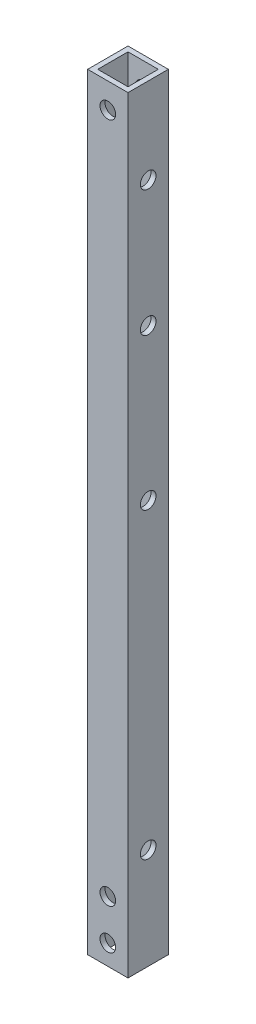
from build123d import *

# Parameters (mm, degrees)
SKETCH_1_W          = 8
SKETCH_1_H          = 8
SKETCH_1_W_2        = 6
SKETCH_1_H_2        = 6
EXTRUDE_1_DEPTH     = 152
SKETCH_2_R          = 1.55
CUT_EXTRUDE_1_DEPTH = 153.262930485
SKETCH_3_R          = 1.55
CUT_EXTRUDE_2_DEPTH = 153.262930485


with BuildPart() as part:
    # 草图1 → 凸台-拉伸1 (new body)
    with BuildSketch(Plane(origin=(0, 0, 0), x_dir=(1, 0, 0), z_dir=(0, 1, 0))):
        Rectangle(SKETCH_1_W, SKETCH_1_H)
        Rectangle(SKETCH_1_W_2, SKETCH_1_H_2, mode=Mode.SUBTRACT)
    extrude(amount=EXTRUDE_1_DEPTH)

    # 草图2 → 切除-拉伸1 (cut, through all)
    with BuildSketch(Plane.XY.offset(4)):
        with Locations((0, 147)):
            Circle(SKETCH_2_R)
        with Locations((0, 4)):
            Circle(SKETCH_2_R)
        with Locations((0, 12)):
            Circle(SKETCH_2_R)
    extrude(amount=-CUT_EXTRUDE_1_DEPTH, mode=Mode.SUBTRACT)

    # 草图3 → 切除-拉伸2 (cut, through all)
    with BuildSketch(Plane(origin=(4, 0, 0), x_dir=(0, 0, -1), z_dir=(1, 0, 0))):
        with Locations((0, 135)):
            Circle(SKETCH_3_R)
        with Locations((0, 20)):
            Circle(SKETCH_3_R)
        with Locations((0, 110)):
            Circle(SKETCH_3_R)
        with Locations((0, 80)):
            Circle(SKETCH_3_R)
    extrude(amount=-CUT_EXTRUDE_2_DEPTH, mode=Mode.SUBTRACT)


solid = part.part
